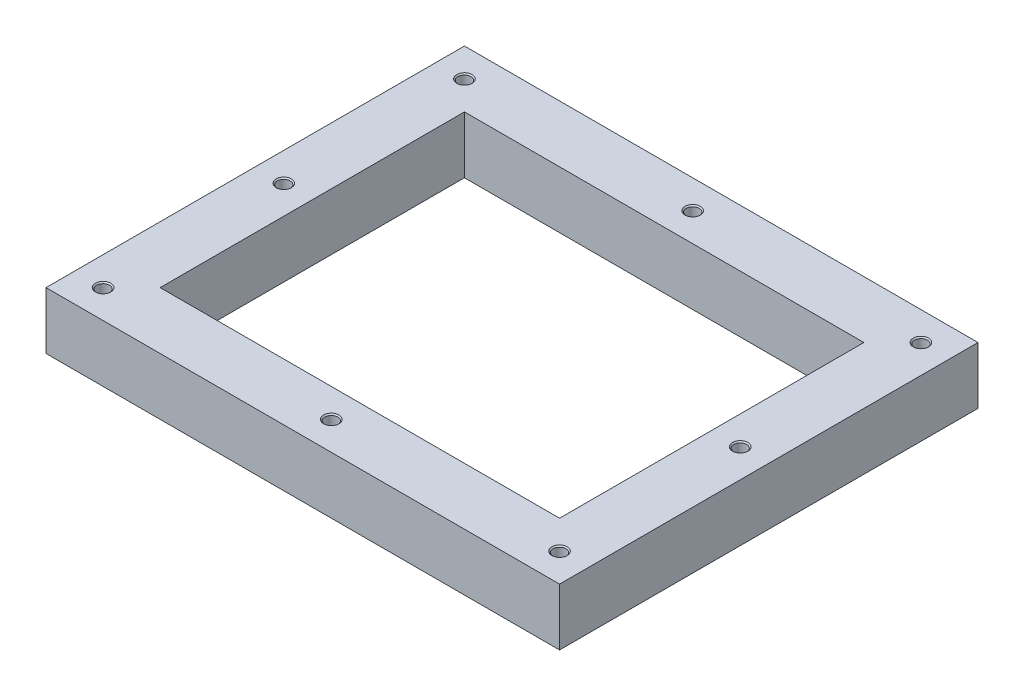
from build123d import *

# Parameters (mm, degrees)
SKETCH1_W                   = 270
SKETCH1_H                   = 220
SKETCH1_W_2                 = 210
SKETCH1_H_2                 = 160
BOSS_EXTRUDE1_DEPTH         = 30
M8_TAPPED_HOLE1_D           = 6.8
M8_TAPPED_HOLE1_DEPTH       = 21.707073895
M8_TAPPED_HOLE1_CSINK_D     = 8.05
M8_TAPPED_HOLE1_CSINK_ANGLE = 90
M8_TAPPED_HOLE1_TIP         = 2.042926105


with BuildPart() as part:
    # Sketch1 → Boss-Extrude1 (new body)
    with BuildSketch(Plane(origin=(0, 0, 0), x_dir=(1, 0, 0), z_dir=(0, 1, 0))):
        Rectangle(SKETCH1_W, SKETCH1_H)
        Rectangle(SKETCH1_W_2, SKETCH1_H_2, mode=Mode.SUBTRACT)
    extrude(amount=BOSS_EXTRUDE1_DEPTH)

    # M8 Tapped Hole1
    with Locations(Plane(origin=(0, 30, 0), x_dir=(1, 0, 0), z_dir=(0, 1, 0))):
        with Locations((0, 95), (-120, 95), (-120, 0), (-120, -95), (0, -95), (120, -95), (120, 95), (120, 0)):
            CounterSinkHole(M8_TAPPED_HOLE1_D / 2, M8_TAPPED_HOLE1_CSINK_D / 2, depth=M8_TAPPED_HOLE1_DEPTH, counter_sink_angle=M8_TAPPED_HOLE1_CSINK_ANGLE)
            with Locations((0, 0, -(M8_TAPPED_HOLE1_DEPTH + M8_TAPPED_HOLE1_TIP / 2))):  # 118° drill point
                Cone(0, M8_TAPPED_HOLE1_D / 2, M8_TAPPED_HOLE1_TIP, mode=Mode.SUBTRACT)


solid = part.part
